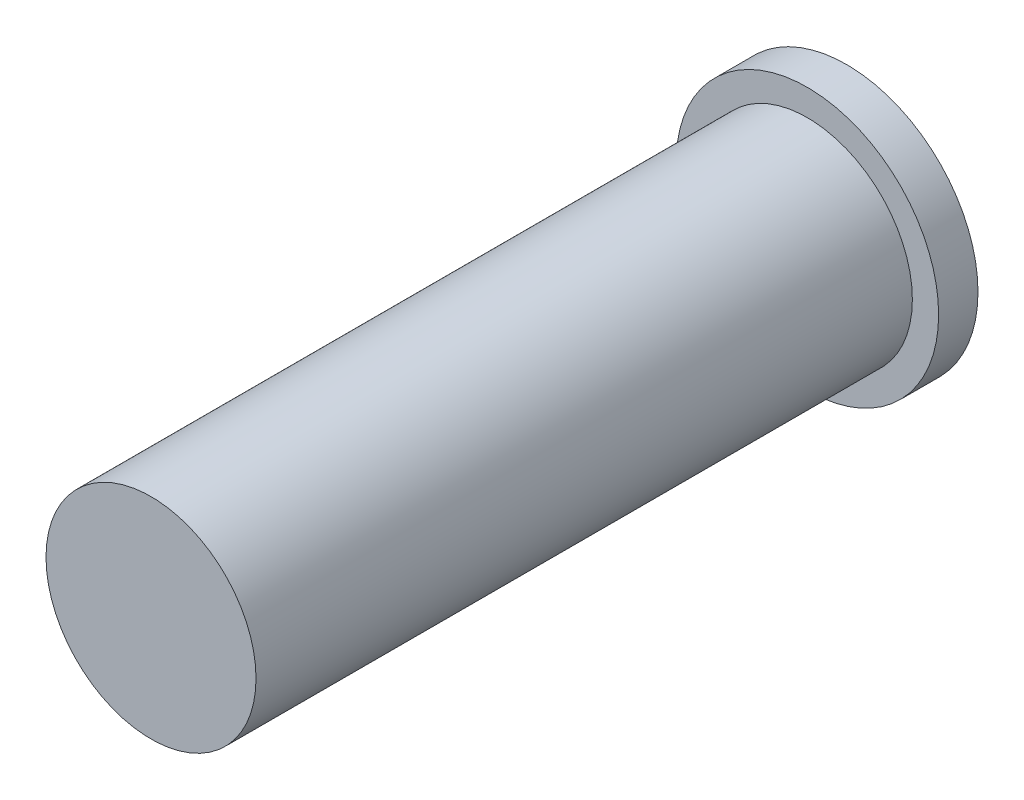
SolidWorks part; units mm, degrees
ref_plane "前视基准面" through (0, 0, 0) normal (0, 0, 1) x (1, 0, 0)
ref_plane "上视基准面" through (0, 0, 0) normal (0, 1, 0) x (1, 0, 0)
ref_plane "右视基准面" through (0, 0, 0) normal (1, 0, 0) x (0, 0, -1)
sketch "草图1" plane through (0, 0, 0) normal (0, 0, 1) x (1, 0, 0)
  circle A0 centre (0, 0) radius 5
  dimension "D1" = 10
extrude "凸台-拉伸1" add sketch "草图1" along normal blind 1.5
sketch "草图2" plane through (0, 0, 1.5) normal (0, 0, 1) x (1, 0, 0)
  circle A0 centre (0, 0) radius 4
  dimension "D1" = 8
extrude "凸台-拉伸2" add sketch "草图2" along normal blind 25
